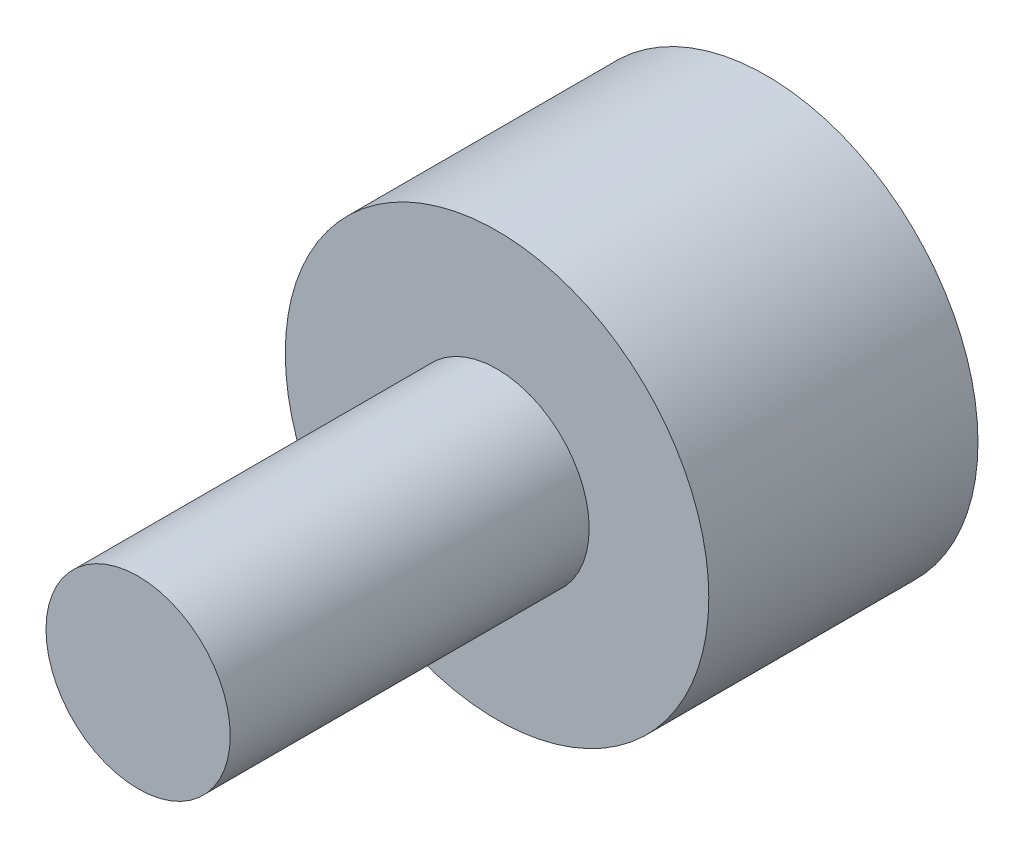
from build123d import *

# Parameters (mm, degrees)
SKETCH_1_R      = 3.54
EXTRUDE_1_DEPTH = 4.5
SKETCH_2_R      = 1.54
EXTRUDE_2_DEPTH = 6


with BuildPart() as part:
    # 草图1 → 凸台-拉伸1 (new body)
    with BuildSketch(Plane.XY):
        Circle(SKETCH_1_R)
    extrude(amount=EXTRUDE_1_DEPTH)

    # 草图2 → 凸台-拉伸2 (add)
    with BuildSketch(Plane.XY.offset(4.5)):
        Circle(SKETCH_2_R)
    extrude(amount=EXTRUDE_2_DEPTH)


solid = part.part
